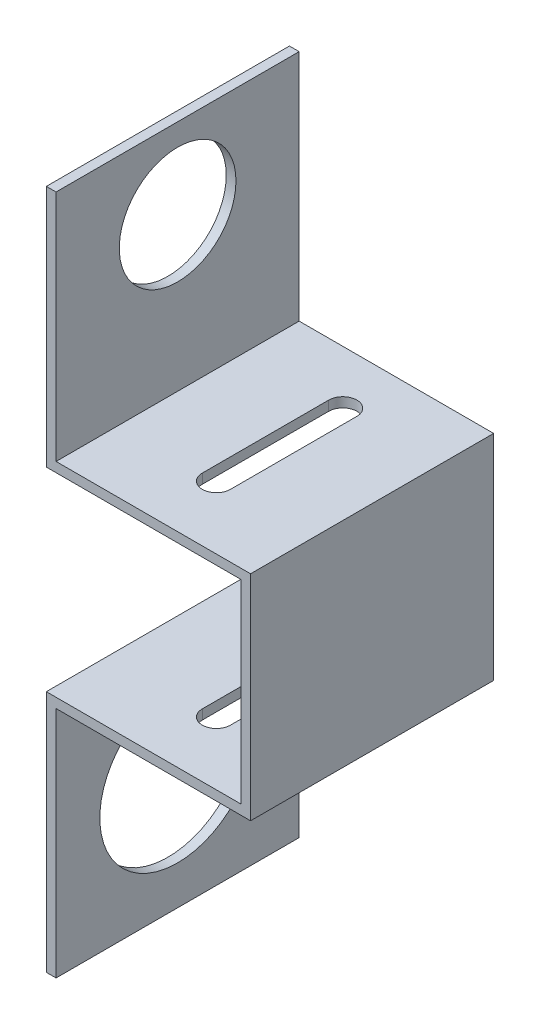
from build123d import *

# Parameters (mm, degrees)
BOSS_EXTRUDE1_DEPTH = 50
CUT_EXTRUDE1_DEPTH  = 50
SKETCH3_R           = 16
CUT_EXTRUDE2_DEPTH  = 50
SKETCH4_R           = 12
CUT_EXTRUDE3_DEPTH  = 50


with BuildPart() as part:
    # Sketch1 → Boss-Extrude1 (new body)
    with BuildSketch(Plane.XY):
        Polygon((0, 50), (0, 0), (40, 0), (40, -40), (0, -40), (0, -90), (2, -90), (2, -42), (42, -42), (42, 2), (2, 2), (2, 50), align=None)
    extrude(amount=BOSS_EXTRUDE1_DEPTH)

    # Sketch2 → Cut-Extrude1 (cut)
    with BuildSketch(Plane(origin=(0, 2, 0), x_dir=(1, 0, 0), z_dir=(0, 1, 0))):
        with BuildLine():
            Line((24.898261367, -11.026648657), (24.898261367, -37.029372299))
            ThreePointArc((24.898261367, -37.029372299), (22, -39.927633667), (19.101738633, -37.029372299))
            Line((19.101738633, -37.029372299), (19.101738633, -11.026648657))
            ThreePointArc((19.101738633, -11.026648657), (22, -8.12838729), (24.898261367, -11.026648657))
        make_face()
    extrude(amount=-CUT_EXTRUDE1_DEPTH, mode=Mode.SUBTRACT)

    # Sketch3 → Cut-Extrude2 (cut)
    with BuildSketch(Plane(origin=(2, 0, 0), x_dir=(0, 0, -1), z_dir=(1, 0, 0))):
        with Locations((-25, -66)):
            Circle(SKETCH3_R)
    extrude(amount=-CUT_EXTRUDE2_DEPTH, mode=Mode.SUBTRACT)

    # Sketch4 → Cut-Extrude3 (cut)
    with BuildSketch(Plane(origin=(2, 0, 0), x_dir=(0, 0, -1), z_dir=(1, 0, 0))):
        with Locations((-25, 33.473514378)):
            Circle(SKETCH4_R)
    extrude(amount=-CUT_EXTRUDE3_DEPTH, mode=Mode.SUBTRACT)


solid = part.part
